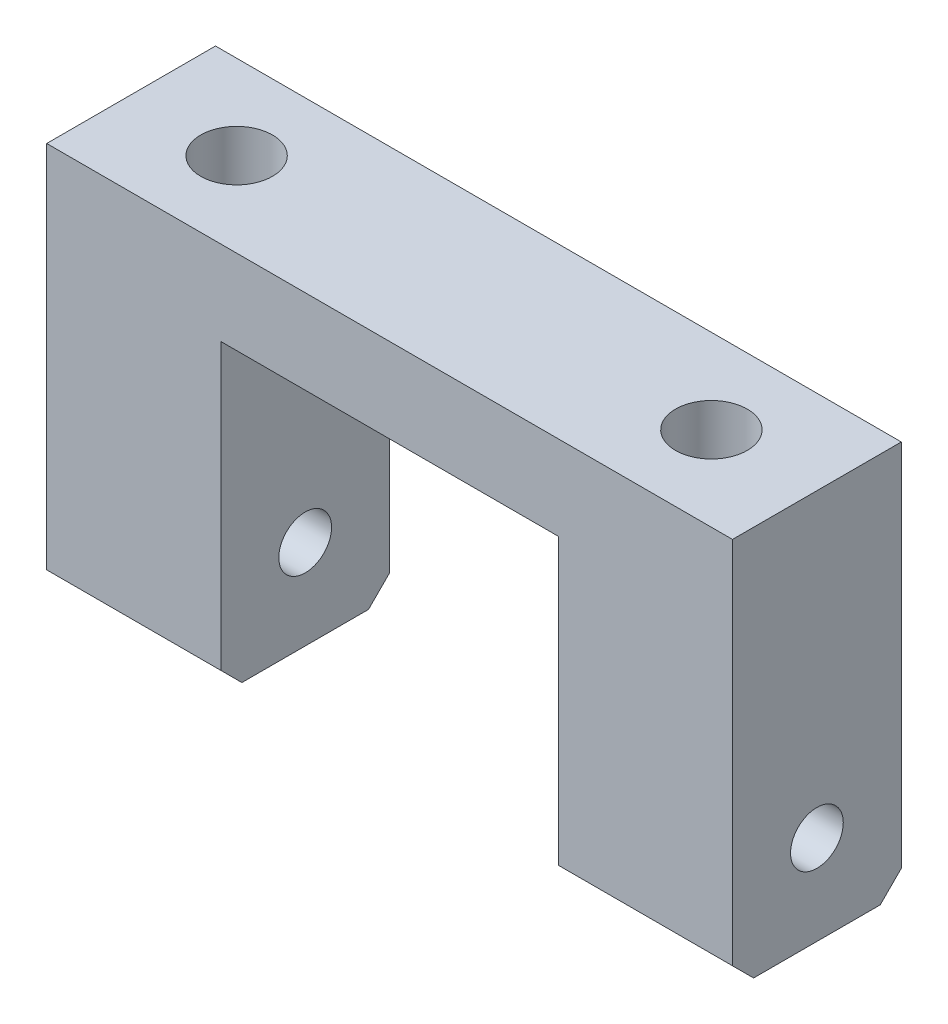
from build123d import *

# Parameters (mm, degrees)
SKETCH_1_W             = 65
SKETCH_1_H             = 37
EXTRUDE_1_DEPTH        = 8
SKETCH_3_W             = 32
SKETCH_3_H             = 29
CUT_EXTRUDE_1_DEPTH    = 41.675545479
HOLE_WIZARD_M6_1_D     = 5
HOLE_WIZARD_M8_2_D     = 6.8
HOLE_WIZARD_M8_2_DEPTH = 22.25
HOLE_WIZARD_M8_2_TIP   = 2.042926105
CHAMFER_1_SIZE         = 2


with BuildPart() as part:
    # 草图1 → 凸台-拉伸1 (new, symmetric)
    with BuildSketch(Plane.XY):
        Rectangle(SKETCH_1_W, SKETCH_1_H)
    extrude(amount=EXTRUDE_1_DEPTH, both=True)

    # 草图3 → 切除-拉伸1 (cut, through all)
    with BuildSketch(Plane.XY.offset(8)):
        with Locations((0, -4)):
            Rectangle(SKETCH_3_W, SKETCH_3_H)
    extrude(amount=-CUT_EXTRUDE_1_DEPTH, mode=Mode.SUBTRACT)

    # M6 螺纹孔1 (through all)
    with Locations(Plane(origin=(32.5, 0, 0), x_dir=(0, 0, -1), z_dir=(1, 0, 0))):
        with Locations((0, -10)):
            Hole(HOLE_WIZARD_M6_1_D / 2)

    # M8 螺纹孔2
    with Locations(Plane(origin=(0, 18.5, 0), x_dir=(1, 0, 0), z_dir=(0, 1, 0))):
        with Locations((-22.5, 0), (22.5, 0)):
            Hole(HOLE_WIZARD_M8_2_D / 2, depth=HOLE_WIZARD_M8_2_DEPTH)
            with Locations((0, 0, -(HOLE_WIZARD_M8_2_DEPTH + HOLE_WIZARD_M8_2_TIP / 2))):  # 118° drill point
                Cone(0, HOLE_WIZARD_M8_2_D / 2, HOLE_WIZARD_M8_2_TIP, mode=Mode.SUBTRACT)

    # 倒角1
    chamfer_1_edges = [part.edges().sort_by_distance(p)[0] for p in [
        (24.25, -18.5, -8),
        (24.25, -18.5, 8),
        (-24.25, -18.5, -8),
        (-24.25, -18.5, 8),
    ]]
    chamfer(chamfer_1_edges, length=CHAMFER_1_SIZE)


solid = part.part
